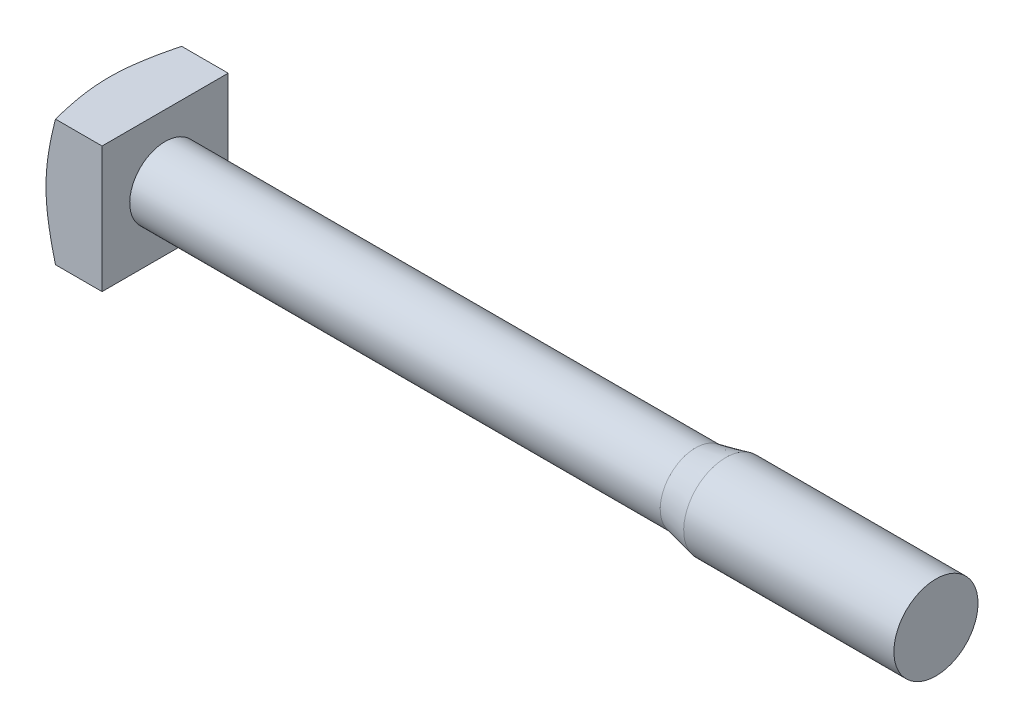
from build123d import *

# Parameters (mm, degrees)
SKETCH1_W      = 18
SKETCH1_H      = 18
BASEHEAD_DEPTH = 8
SKETCH2_R      = 6
BASEBODY_DEPTH = 110


with BuildPart() as part:
    # Sketch1 → BaseHead (new body)
    with BuildSketch(Plane(origin=(0, 0, 0), x_dir=(0, 0, -1), z_dir=(1, 0, 0))):
        Rectangle(SKETCH1_W, SKETCH1_H)
    extrude(amount=BASEHEAD_DEPTH)

    # Sketch4 → HeadChamfer (revolve, cut)
    with BuildSketch(Plane(origin=(-7.181436497, -8, 8), x_dir=(-1, 0, 0), z_dir=(0, -0.7071067811865485, -0.7071067811865466))):
        Polygon((-7.181436497, 20.313708499), (-7.181436497, 24.04163056), (-8.538289163, 24.04163056), align=None)
    revolve(axis=Axis((8.946843605, 0, 0), (-1, 0, 0)), mode=Mode.SUBTRACT)

    # Sketch2 → BaseBody (add)
    with BuildSketch(Plane(origin=(8, 0, 0), x_dir=(0, 0, -1), z_dir=(1, 0, 0))):
        Circle(SKETCH2_R)
    extrude(amount=BASEBODY_DEPTH)

    # Sketch5 → Cut-Revolve1 (revolve, cut)
    with BuildSketch(Plane(origin=(-43.209051362, 5, 0), x_dir=(-1, 0, 0), z_dir=(0, 0, 1))):
        Polygon((-131.209051362, 11), (-51.209051362, 11), (-51.209051362, 10.053), (-126.909051362, 10.053), align=None)
    revolve(axis=Axis((-3.790948638, 0, 0), (1, 0, 0)), mode=Mode.SUBTRACT)


solid = part.part
